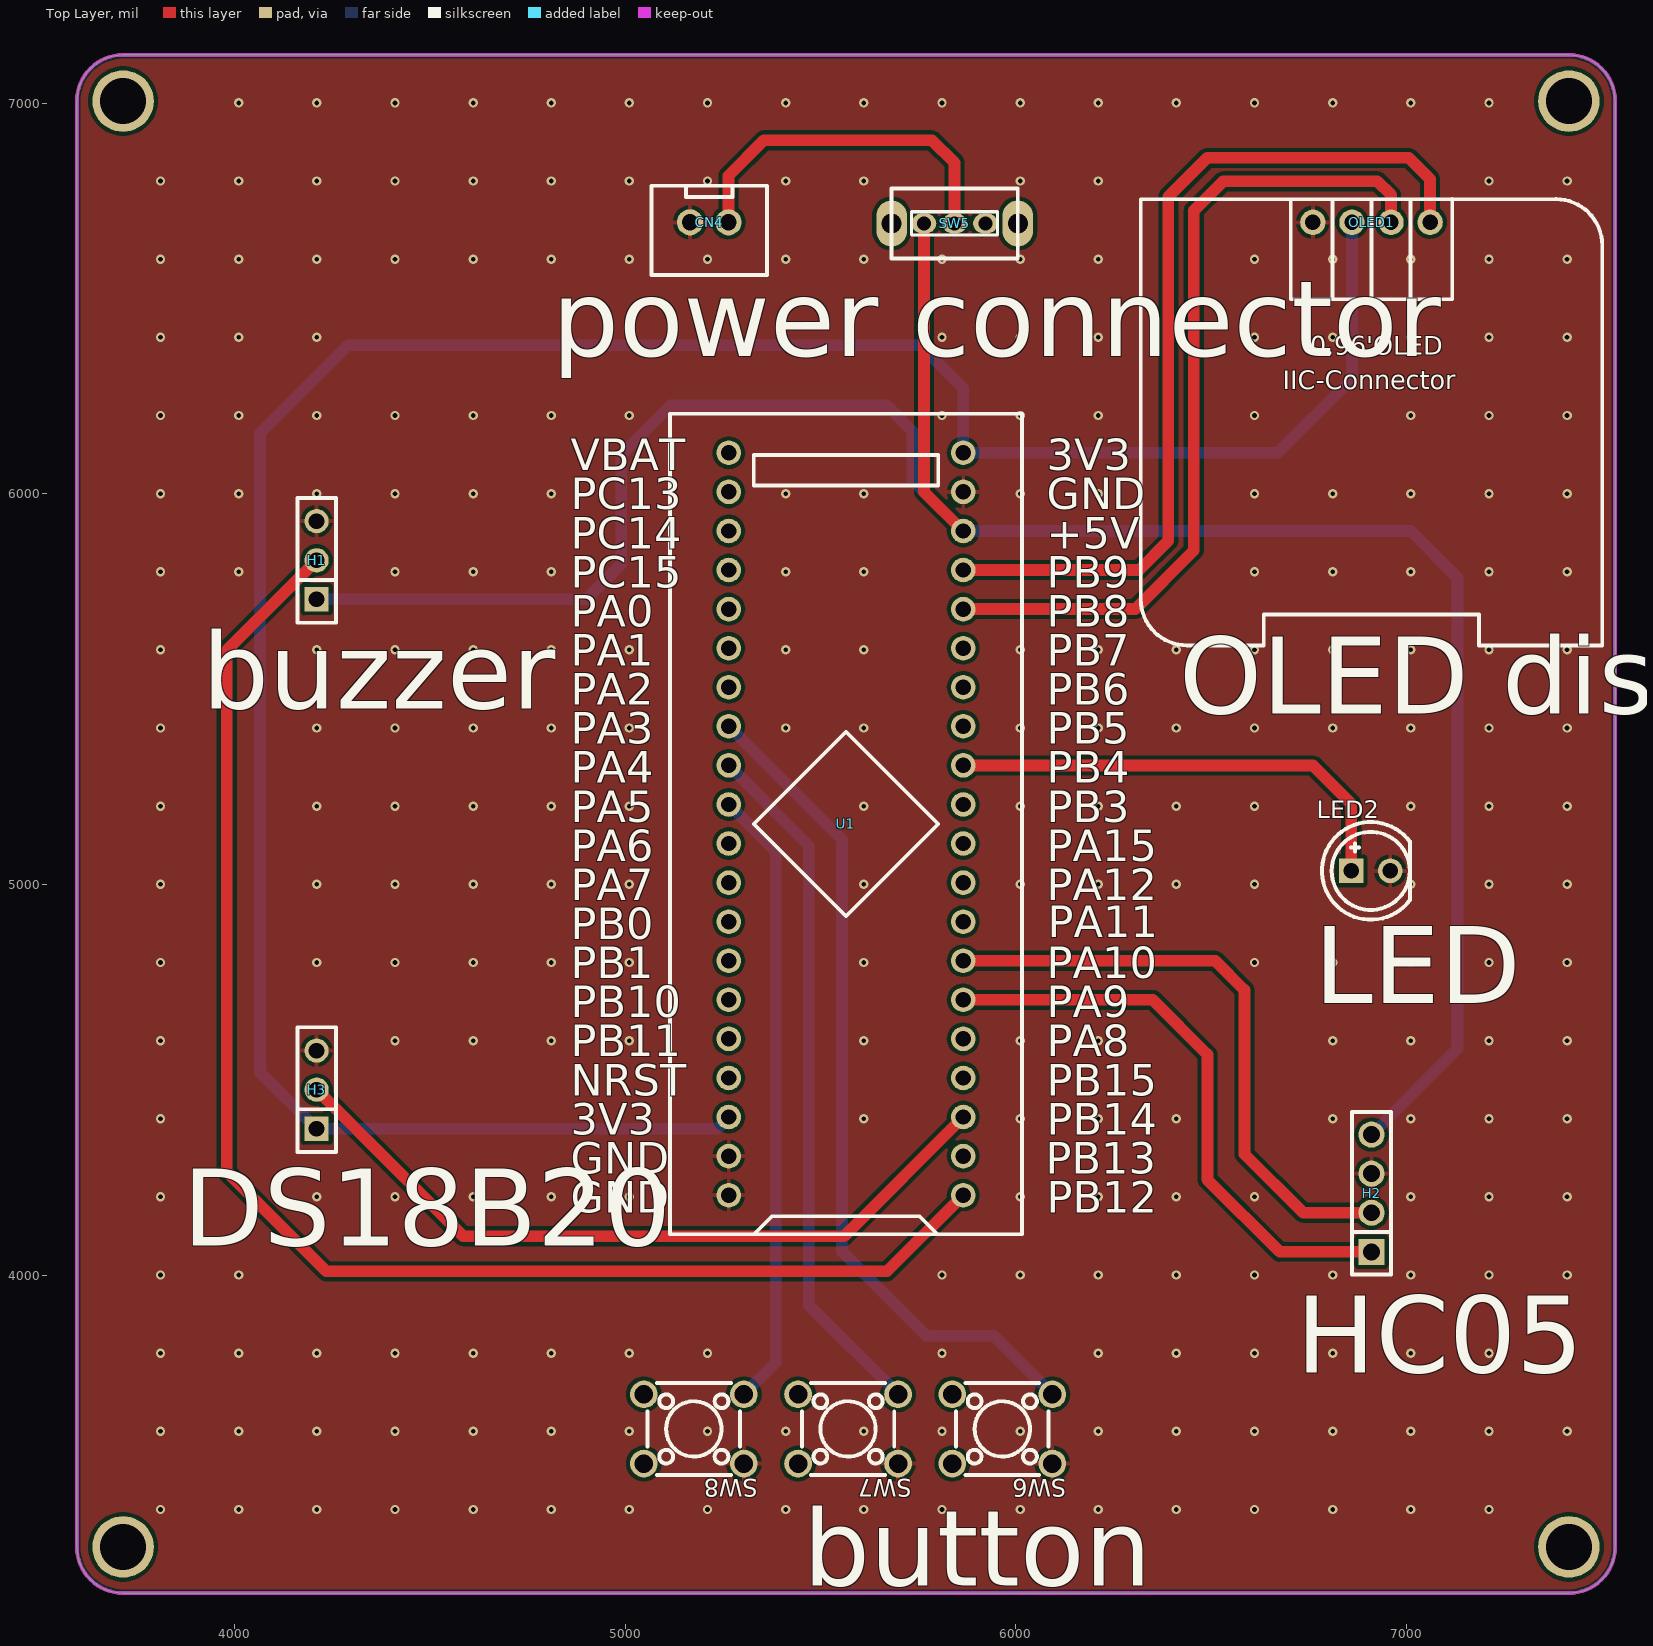
[diagram p0: Top Layer view]
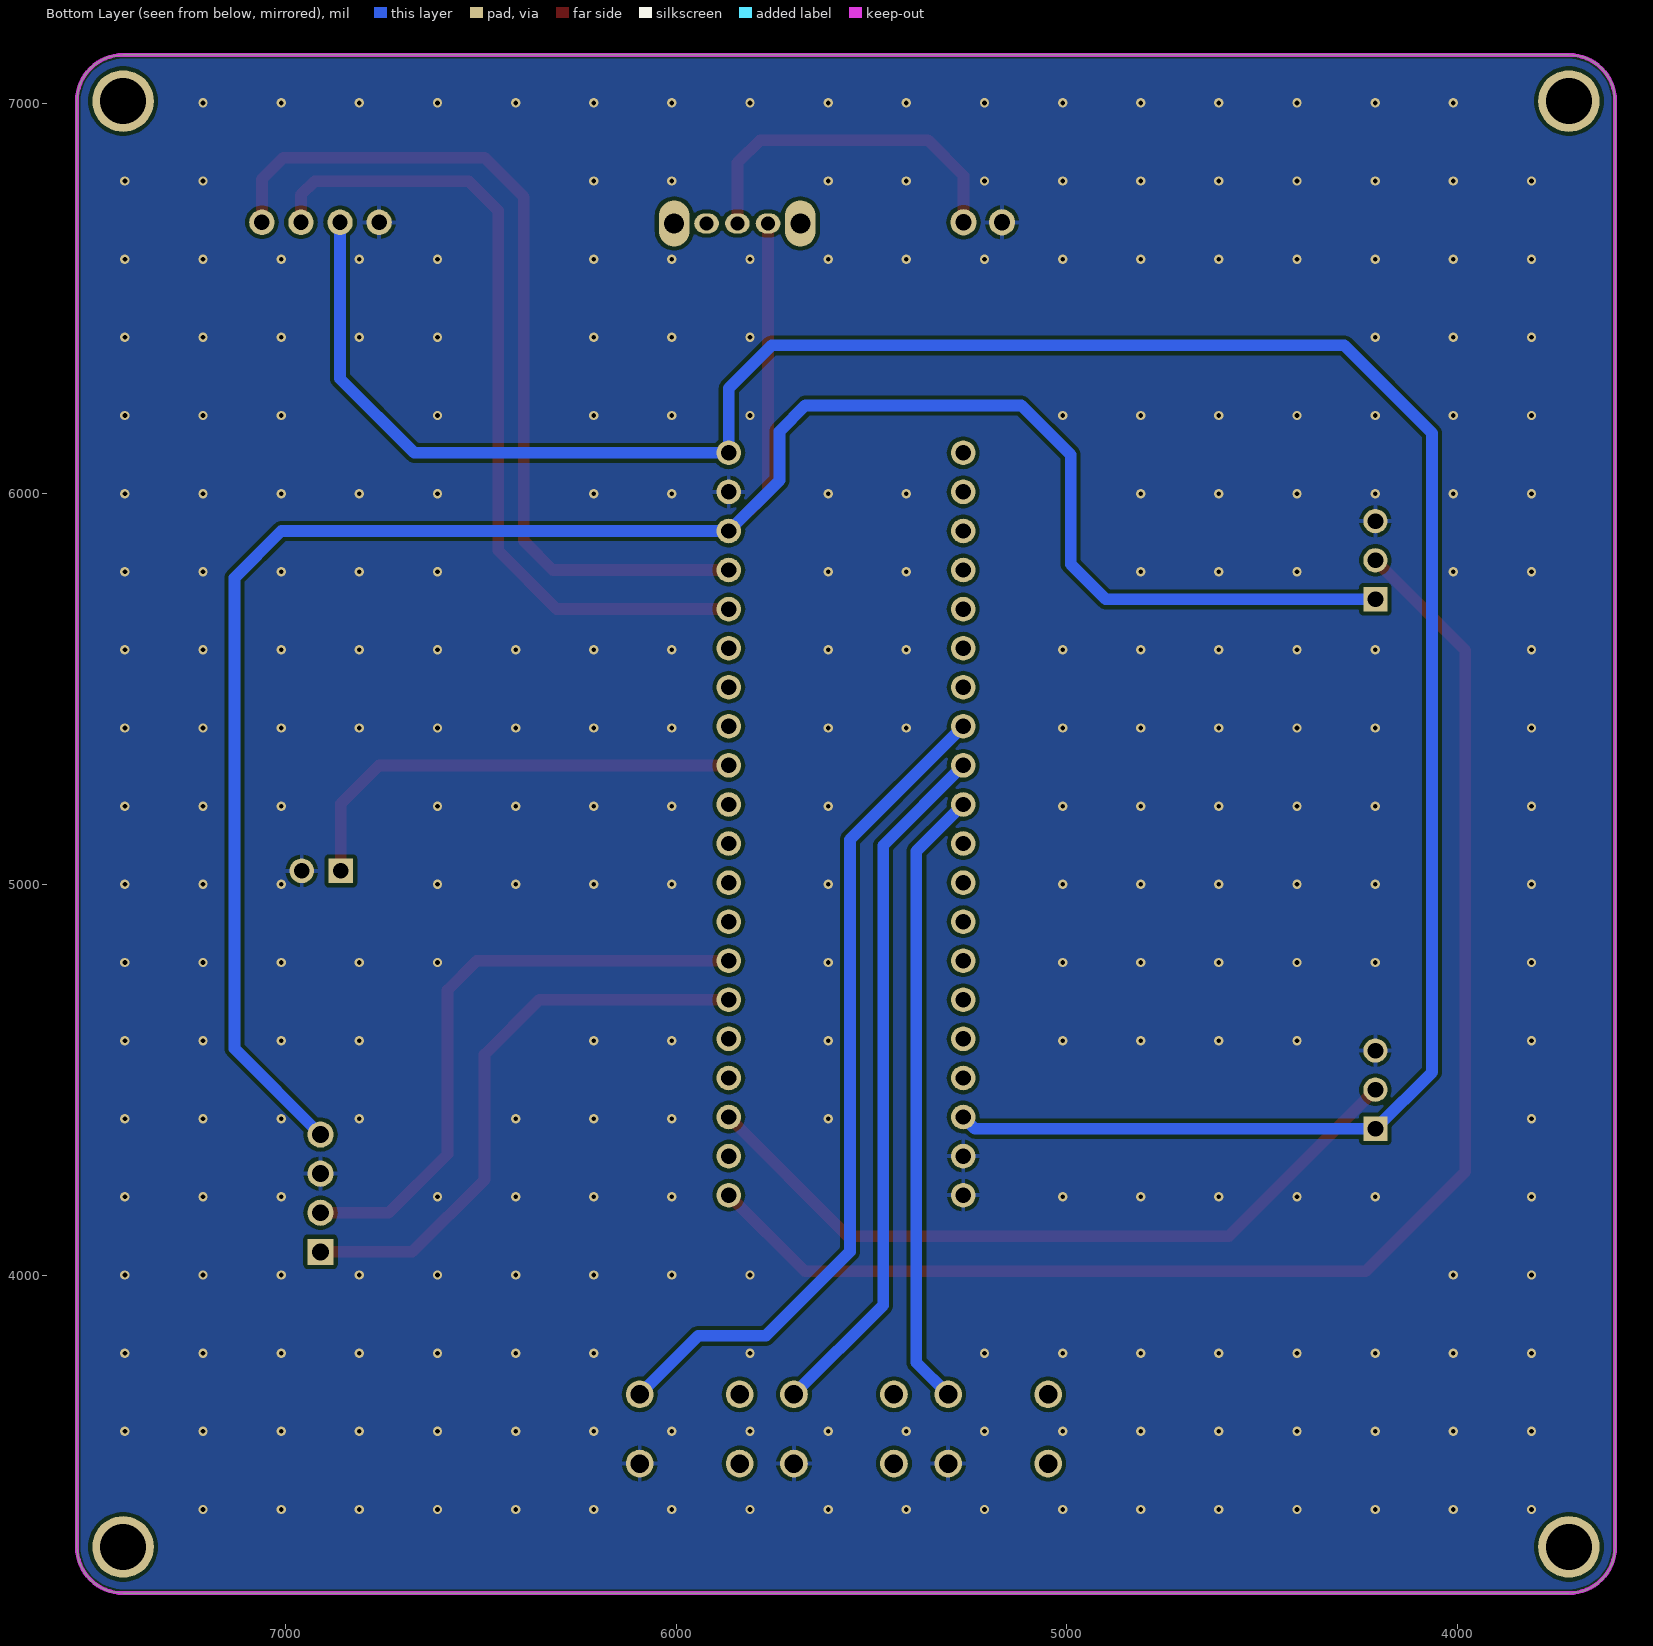
[diagram p1: Bottom Layer view, seen from below]
# Altium PCB MISC89015.pcbdoc
Units mil, origin at the board's own origin, x right, y up, seen from the top; angles counter-clockwise.
Board outline 3937.01 x 3937.01 mil, 2 copper layers (Top Layer, Bottom Layer), stack 62.206 mil thick; 11 components, 38 nets, 79 pads, 271 vias.

## Layer stack, top to bottom
Top Solder Mask Layer: solder mask 0.394, Dk 3.3
Top Layer: signal copper 1.379
Dielectric1: surface 59.449, FR4, Dk 4.5
Bottom Layer: signal copper 1.378
Bottom Solder Mask Layer: solder mask 0.394, Dk 3.3

## Board outline
3714.61,7123.5 ccw(c3714.61,7005.39) 3596.5,7005.39 3596.5,3304.61 ccw(c3714.61,3304.61) 3714.61,3186.5 7415.39,3186.5 ccw(c7415.39,3304.61) 7533.5,3304.61 7533.5,7005.39 ccw(c7415.39,7005.39) 7415.39,7123.5 3714.61,7123.5

## Design rules (kind name [scope] priority, off if disabled: settings)
BoardOutlineClearance copperThickness2oz_1 [All] p2 off: genericclearance=7.99 ignorepadtopadclearanceinfootprint=FALSE except(0: Arc-SplitContinuation Track-SplitContinuation SMDPad-SplitContinuation THPad-SplitContinuation Via-SplitContinuation Fill-SplitContinuation Region-SplitContinuation Poly-SplitContinuation Text-SplitContinuation Hole-SplitContinuation; 5.98: Arc-CutoutEdge Track-CutoutEdge SMDPad-CutoutEdge THPad-CutoutEdge Via-CutoutEdge Text-CutoutEdge; 6.9: Hole-OutlineEdge Hole-CutoutEdge; 10: Poly-OutlineEdge Poly-CutoutEdge; 11.81: Arc-OutlineEdge Track-OutlineEdge SMDPad-OutlineEdge THPad-OutlineEdge Via-OutlineEdge Fill-OutlineEdge Region-OutlineEdge Text-OutlineEdge Fill-CutoutEdge Region-CutoutEdge)
BoardOutlineClearance Plane_innerPlane_1 [All] p4 off: genericclearance=4.02 ignorepadtopadclearanceinfootprint=FALSE except(0: Arc-SplitContinuation Track-SplitContinuation SMDPad-SplitContinuation THPad-SplitContinuation Via-SplitContinuation Fill-SplitContinuation Region-SplitContinuation Poly-SplitContinuation Text-SplitContinuation Hole-SplitContinuation; 5.98: Arc-CutoutEdge Track-CutoutEdge SMDPad-CutoutEdge THPad-CutoutEdge Via-CutoutEdge Text-CutoutEdge; 6.9: Hole-OutlineEdge Hole-CutoutEdge; 10: Poly-OutlineEdge Poly-CutoutEdge; 11.81: Arc-OutlineEdge Track-OutlineEdge SMDPad-OutlineEdge THPad-OutlineEdge Via-OutlineEdge Fill-OutlineEdge Region-OutlineEdge Text-OutlineEdge Fill-CutoutEdge Region-CutoutEdge)
BoardOutlineClearance Copper_copperRegion_1 [All] p6 off: genericclearance=4.02 ignorepadtopadclearanceinfootprint=FALSE except(0: Arc-SplitContinuation Track-SplitContinuation SMDPad-SplitContinuation THPad-SplitContinuation Via-SplitContinuation Fill-SplitContinuation Region-SplitContinuation Poly-SplitContinuation Text-SplitContinuation Hole-SplitContinuation; 5.98: Arc-CutoutEdge Track-CutoutEdge SMDPad-CutoutEdge THPad-CutoutEdge Via-CutoutEdge Text-CutoutEdge; 6.9: Hole-OutlineEdge Hole-CutoutEdge; 10: Poly-OutlineEdge Poly-CutoutEdge; 11.81: Arc-OutlineEdge Track-OutlineEdge SMDPad-OutlineEdge THPad-OutlineEdge Via-OutlineEdge Fill-OutlineEdge Region-OutlineEdge Text-OutlineEdge Fill-CutoutEdge Region-CutoutEdge)
BoardOutlineClearance Copper_copperRegion_copperThickness1oz_1 [All] p8 off: genericclearance=4.02 ignorepadtopadclearanceinfootprint=FALSE except(0: Arc-SplitContinuation Track-SplitContinuation SMDPad-SplitContinuation THPad-SplitContinuation Via-SplitContinuation Fill-SplitContinuation Region-SplitContinuation Poly-SplitContinuation Text-SplitContinuation Hole-SplitContinuation; 5.98: Arc-CutoutEdge Track-CutoutEdge SMDPad-CutoutEdge THPad-CutoutEdge Via-CutoutEdge Text-CutoutEdge; 6.9: Hole-OutlineEdge Hole-CutoutEdge; 10: Poly-OutlineEdge Poly-CutoutEdge; 11.81: Arc-OutlineEdge Track-OutlineEdge SMDPad-OutlineEdge THPad-OutlineEdge Via-OutlineEdge Fill-OutlineEdge Region-OutlineEdge Text-OutlineEdge Fill-CutoutEdge Region-CutoutEdge)
BoardOutlineClearance Copper_copperRegion_Copper_copperRegion_1 [All] p10 off: genericclearance=4.02 ignorepadtopadclearanceinfootprint=FALSE except(0: Arc-SplitContinuation Track-SplitContinuation SMDPad-SplitContinuation THPad-SplitContinuation Via-SplitContinuation Fill-SplitContinuation Region-SplitContinuation Poly-SplitContinuation Text-SplitContinuation Hole-SplitContinuation; 5.98: Arc-CutoutEdge Track-CutoutEdge SMDPad-CutoutEdge THPad-CutoutEdge Via-CutoutEdge Text-CutoutEdge; 6.9: Hole-OutlineEdge Hole-CutoutEdge; 10: Poly-OutlineEdge Poly-CutoutEdge; 11.81: Arc-OutlineEdge Track-OutlineEdge SMDPad-OutlineEdge THPad-OutlineEdge Via-OutlineEdge Fill-OutlineEdge Region-OutlineEdge Text-OutlineEdge Fill-CutoutEdge Region-CutoutEdge)
BoardOutlineClearance copperThickness1oz_1 [All] p12: genericclearance=4.02 ignorepadtopadclearanceinfootprint=FALSE except(0: Arc-SplitContinuation Track-SplitContinuation SMDPad-SplitContinuation THPad-SplitContinuation Via-SplitContinuation Fill-SplitContinuation Region-SplitContinuation Poly-SplitContinuation Text-SplitContinuation Hole-SplitContinuation; 5.98: Arc-CutoutEdge Track-CutoutEdge SMDPad-CutoutEdge THPad-CutoutEdge Via-CutoutEdge Text-CutoutEdge; 6.9: Hole-OutlineEdge Hole-CutoutEdge; 10: Poly-OutlineEdge Poly-CutoutEdge; 11.81: Arc-OutlineEdge Track-OutlineEdge SMDPad-OutlineEdge THPad-OutlineEdge Via-OutlineEdge Fill-OutlineEdge Region-OutlineEdge Text-OutlineEdge Fill-CutoutEdge Region-CutoutEdge)
Clearance copperThickness2oz [All] p1 off: gap=7.99 ignorepadtopadclearanceinfootprint=FALSE except(5.98: SMDPad-Track SMDPad-SMDPad THPad-Track SMDPad-THPad THPad-THPad Track-Via SMDPad-Via THPad-Via Via-Via Fill-SMDPad Region-SMDPad Fill-THPad Region-THPad Fill-Via Region-Via Fill-Fill Fill-Region Region-Region Arc-Track Arc-SMDPad Arc-THPad Arc-Via Fill-Arc Region-Arc Arc-Arc Text-Track SMDPad-Text Text-THPad Text-Via Fill-Text Region-Text Arc-Text Text-Text; 6.9: Hole-Track Hole-SMDPad Hole-THPad Hole-Via Fill-Hole Region-Hole Hole-Arc Hole-Text; 10: Poly-Track Poly-SMDPad Poly-THPad Poly-Via Poly-Fill Poly-Region Poly-Poly Poly-Arc Poly-Text Poly-Hole; 11.81: Fill-Track Region-Track)
Clearance Plane_innerPlane [All] p3 off: gap=4.02 ignorepadtopadclearanceinfootprint=FALSE except(5.98: SMDPad-Track SMDPad-SMDPad THPad-Track SMDPad-THPad THPad-THPad Track-Via SMDPad-Via THPad-Via Via-Via Fill-SMDPad Region-SMDPad Fill-THPad Region-THPad Fill-Via Region-Via Fill-Fill Fill-Region Region-Region Arc-Track Arc-SMDPad Arc-THPad Arc-Via Fill-Arc Region-Arc Arc-Arc Text-Track SMDPad-Text Text-THPad Text-Via Fill-Text Region-Text Arc-Text Text-Text; 6.9: Hole-Track Hole-SMDPad Hole-THPad Hole-Via Fill-Hole Region-Hole Hole-Arc Hole-Text; 10: Poly-Track Poly-SMDPad Poly-THPad Poly-Via Poly-Fill Poly-Region Poly-Poly Poly-Arc Poly-Text Poly-Hole; 11.81: Fill-Track Region-Track)
Clearance Copper_copperRegion [All] p5 off: gap=4.02 ignorepadtopadclearanceinfootprint=FALSE except(5.98: SMDPad-Track SMDPad-SMDPad THPad-Track SMDPad-THPad THPad-THPad Track-Via SMDPad-Via THPad-Via Via-Via Fill-SMDPad Region-SMDPad Fill-THPad Region-THPad Fill-Via Region-Via Fill-Fill Fill-Region Region-Region Arc-Track Arc-SMDPad Arc-THPad Arc-Via Fill-Arc Region-Arc Arc-Arc Text-Track SMDPad-Text Text-THPad Text-Via Fill-Text Region-Text Arc-Text Text-Text; 6.9: Hole-Track Hole-SMDPad Hole-THPad Hole-Via Fill-Hole Region-Hole Hole-Arc Hole-Text; 10: Poly-Track Poly-SMDPad Poly-THPad Poly-Via Poly-Fill Poly-Region Poly-Poly Poly-Arc Poly-Text Poly-Hole; 11.81: Fill-Track Region-Track)
Clearance Copper_copperRegion_copperThickness1oz [All] p7 off: gap=4.02 ignorepadtopadclearanceinfootprint=FALSE except(5.98: SMDPad-Track SMDPad-SMDPad THPad-Track SMDPad-THPad THPad-THPad Track-Via SMDPad-Via THPad-Via Via-Via Fill-SMDPad Region-SMDPad Fill-THPad Region-THPad Fill-Via Region-Via Fill-Fill Fill-Region Region-Region Arc-Track Arc-SMDPad Arc-THPad Arc-Via Fill-Arc Region-Arc Arc-Arc Text-Track SMDPad-Text Text-THPad Text-Via Fill-Text Region-Text Arc-Text Text-Text; 6.9: Hole-Track Hole-SMDPad Hole-THPad Hole-Via Fill-Hole Region-Hole Hole-Arc Hole-Text; 10: Poly-Track Poly-SMDPad Poly-THPad Poly-Via Poly-Fill Poly-Region Poly-Poly Poly-Arc Poly-Text Poly-Hole; 11.81: Fill-Track Region-Track)
Clearance Copper_copperRegion_Copper_copperRegion [All] p9 off: gap=4.02 ignorepadtopadclearanceinfootprint=FALSE except(5.98: SMDPad-Track SMDPad-SMDPad THPad-Track SMDPad-THPad THPad-THPad Track-Via SMDPad-Via THPad-Via Via-Via Fill-SMDPad Region-SMDPad Fill-THPad Region-THPad Fill-Via Region-Via Fill-Fill Fill-Region Region-Region Arc-Track Arc-SMDPad Arc-THPad Arc-Via Fill-Arc Region-Arc Arc-Arc Text-Track SMDPad-Text Text-THPad Text-Via Fill-Text Region-Text Arc-Text Text-Text; 6.9: Hole-Track Hole-SMDPad Hole-THPad Hole-Via Fill-Hole Region-Hole Hole-Arc Hole-Text; 10: Poly-Track Poly-SMDPad Poly-THPad Poly-Via Poly-Fill Poly-Region Poly-Poly Poly-Arc Poly-Text Poly-Hole; 11.81: Fill-Track Region-Track)
Clearance copperThickness1oz [All] p11: gap=4.02 ignorepadtopadclearanceinfootprint=FALSE except(5.98: SMDPad-Track SMDPad-SMDPad THPad-Track SMDPad-THPad THPad-THPad Track-Via SMDPad-Via THPad-Via Via-Via Fill-SMDPad Region-SMDPad Fill-THPad Region-THPad Fill-Via Region-Via Fill-Fill Fill-Region Region-Region Arc-Track Arc-SMDPad Arc-THPad Arc-Via Fill-Arc Region-Arc Arc-Arc Text-Track SMDPad-Text Text-THPad Text-Via Fill-Text Region-Text Arc-Text Text-Text; 6.9: Hole-Track Hole-SMDPad Hole-THPad Hole-Via Fill-Hole Region-Hole Hole-Arc Hole-Text; 10: Poly-Track Poly-SMDPad Poly-THPad Poly-Via Poly-Fill Poly-Region Poly-Poly Poly-Arc Poly-Text Poly-Hole; 11.81: Fill-Track Region-Track)
DiffPairsRouting differentialPair [All] p1: maxlimit=6 minlimit=6 mostfreqgap=6 toplayer_minwidth=5 toplayer_prefwidth=10 toplayer_maxwidth=100 toplayer_mingap=6 toplayer_prefgap=6 toplayer_maxgap=6 bottomlayer_minwidth=5 bottomlayer_prefwidth=10 bottomlayer_maxwidth=100 bottomlayer_mingap=6 bottomlayer_prefgap=6 bottomlayer_maxgap=6 maxuncoupledlength=10
HoleToHoleClearance otherClearance [All] p1: gap=11.81 allowstackedmicrovias=TRUE
Length netLength [All] p1: minlimit=0 maxlimit=0
PasteMaskExpansion pasteMaskExpansion [All] p1: expansion=0
PlaneConnect innerPlane [All] p1: planeconnectstyle=Relief reliefexpansion=20 reliefentries=4 reliefconductorwidth=10 reliefairgap=10
PolygonConnect copperRegion_copperThickness1oz [All] p1 off: connectstyle=Relief reliefconductorwidth=10 reliefentries=4 polygonreliefangle="90 Angle" airgapwidth=10 via.connectstyle=Relief via.reliefconductorwidth=10 via.reliefentries=4 via.polygonreliefangle="90 Angle" via.airgapwidth=10
PolygonConnect copperRegion_Copper_copperRegion [All] p2 off: connectstyle=Relief reliefconductorwidth=10 reliefentries=4 polygonreliefangle="90 Angle" airgapwidth=10 via.connectstyle=Relief via.reliefconductorwidth=10 via.reliefentries=4 via.polygonreliefangle="90 Angle" via.airgapwidth=10
PolygonConnect copperRegion [All] p3: connectstyle=Relief reliefconductorwidth=10 reliefentries=4 polygonreliefangle="90 Angle" airgapwidth=10 via.connectstyle=Relief via.reliefconductorwidth=10 via.reliefentries=4 via.polygonreliefangle="90 Angle" via.airgapwidth=10
RoutingVias viaSize [All] p1: holewidth=12.01 width=24.02 viastyle="Through Hole" minholewidth=11.81 minwidth=19.68 maxholewidth=248.03 maxwidth=393.7
SolderMaskExpansion solderMaskExpansion [IsVia] p1: expansion=-1000 istentingtop=TRUE
SolderMaskExpansion solderMaskExpansion [All] p2: expansion=2 istentingtop=FALSE
Width copperThickness2oz_2 [All] p1 off: maxlimit=100 minlimit=8 preferedwidth=10
Width copperThickness1oz_2 [All] p2: maxlimit=100 minlimit=5 preferedwidth=10

## Components (designator, comment, footprint, x,y, rotation, side; value= is the part's Value field where it differs from the comment)
CN4 "XH2.54*2P_THT" CONN-TH_2P-P2.50-XH2.54-2P 5215,6695 r0 top
H1 "" HDR-TH_3P-P2.54-V-F 4210,5830 r90 top
H2 "" HDR-TH_4P-P2.54-V-F 6910,4210 r90 top
H3 "" HDR-TH_3P-P2.54-V-F 4210,4475 r90 top
LED2 "" LED-TH_5mm 6908.03,5035 r0 top
OLED1 "" 0.96OLED_4P 6910,6695 r0 top
SW5 "" 拨动开关 5837.9,6692.05 r0 top
SW6 "" SW-TH_4P-L6.0-W6.0-P4.50-LS6.5 5965,3606.64 r180 top
SW7 "" SW-TH_4P-L6.0-W6.0-P4.50-LS6.5 5570.29,3606.64 r180 top
SW8 "" SW-TH_4P-L6.0-W6.0-P4.50-LS6.5 5175.57,3606.64 r180 top
U1 "STM32F103C8T6-Card" CONN-TH_L53.3-W22.9_STM32F103C8T6-CARD 5565,5155 r90 top

## Footprints (in the part's own frame and the unit in brackets; to place one, negate y for a bottom-side part, rotate by r counter-clockwise, add the part's x,y. Pads: shape width x height; smd on the part's side, far side on the other; paste and mask are expansions set on the pad)
0.96OLED_4P [mm]
  round 1.65 hole 1 copper offset 0,0: 1(-3.81,-0.001) 2(-1.27,0.002) 3(1.27,0.002) 4(3.81,0.002)
  silkscreen extent -15,-27.5 15,1.5
CONN-TH_2P-P2.50-XH2.54-2P [mm]
  round 1.7 hole 1.05 paste+0 mask+0.05: 1(1.25,0) 2(-1.25,0)
  silkscreen extent -3.75,-3.42 3.75,2.37
CONN-TH_L53.3-W22.9_STM32F103C8T6-CARD [mm]
  round 1.6 hole 1: 1(-24.13,-7.62) 2(-21.59,-7.62) 3(-19.05,-7.62) 4(-16.51,-7.62) 5(-13.97,-7.62) 6(-11.43,-7.62) 7(-8.89,-7.62) 8(-6.35,-7.62) 9(-3.81,-7.62) 10(-1.27,-7.62) 11(1.27,-7.62) 12(3.81,-7.62) 13(6.35,-7.62) 14(8.89,-7.62) 15(11.43,-7.62) 16(13.97,-7.62) 17(16.51,-7.62) 18(19.05,-7.62) 19(21.59,-7.62) 20(24.13,-7.62) 21(24.13,7.62) 22(21.59,7.62) 23(19.05,7.62) 24(16.51,7.62) 25(13.97,7.62) 26(11.43,7.62) 27(8.89,7.62) 28(6.35,7.62) 29(3.81,7.62) 30(1.27,7.62) 31(-1.27,7.62) 32(-3.81,7.62) 33(-6.35,7.62) 34(-8.89,7.62) 35(-11.43,7.62) 36(-13.97,7.62) 37(-16.51,7.62) 38(-19.05,7.62) 39(-21.59,7.62) 40(-24.13,7.62)
  silkscreen extent -26.67,-11.43 26.67,11.43
HDR-TH_3P-P2.54-V-F [mil]
  rect 62x62 hole 40.16: 1(-100,0)
  round 62 hole 40.16: 2(0,0) 3(100,0)
  silkscreen extent -160,-49 160,49
HDR-TH_4P-P2.54-V-F [mm]
  rect 1.7x1.7 hole 1.1: 1(-3.81,0)
  round 1.7 hole 1.1: 2(-1.27,0) 3(1.27,0) 4(3.81,0)
  silkscreen extent -5.29,-1.27 5.29,1.27
LED-TH_5mm [mm]
  rect 1.6x1.6 hole 1 paste+0 mask+0.051: 1(-1.27,0)
  round 1.6 hole 1 paste+0 mask+0.051: 2(1.27,0)
  silkscreen extent -3.17,-3.17 2.54,3.17
SW-TH_4P-L6.0-W6.0-P4.50-LS6.5 [mm]
  round 1.8 hole 1.2: 1(-3.25,2.25) 2(3.25,2.25) 3(-3.25,-2.25) 4(3.25,-2.25)
  silkscreen extent -3,-3 3,3
拨动开关 [mil]
  oval 63x51.2 hole 35.4 paste+0 mask+2: 1(-73.4,0) 2(5,0) 3(84,0)
  oval 78.7x118.1 hole 51.2 paste+0 mask+2: 4(166.7,0) 5(-156.1,0)
  silkscreen extent -156,-90 167,90

## Free pads (board coordinates)
  round 157.48 hole 118.11: 1(3714.61,7005.39) 1(3714.61,3304.61) 1(7415.39,7005.39) 1(7415.39,3304.61)

## Via types
v1: diameter 24.02, hole 12, Top Layer to Bottom Layer, 271 vias

## Nets (pads, with @x,y where several pads share a name; then routed paths per layer and width w, separated by ;. In a path a pad name is that pad's centre, name@x,y a point inside that pad or via, vN(x,y) a via of type N, cw(c..) or ccw(c..) an arc to the next point about the centre after c; other vN are vias at no path point)
$1N17118: CN4.1 SW5.2 | length 914.5
  Top Layer w30: CN4.1 5264.22,6814.22 5355,6905 5785,6905 5842.9,6847.1 SW5.2
+5V: H1.1 H2.4 SW5.1 U1.18 | length 5890.3
  Top Layer w30: SW5.1 5764.5,6005.5 U1.18
  Bottom Layer w30: H1.1 4900,5730 4990,5820 4990,6100 5116.21,6226.21 5668.79,6226.21 5735,6160 5735,6035 U1.18 7010,5905 7130,5785 7130,4580 H2.4
GND: CN4.2 H1.3 H2.3 H3.3 LED2.2 OLED1.1 SW6.1 SW7.1 SW8.1 U1.19 U1.39 U1.40
  other v1: 3810.6,3400.6 4010.6,3400.6 4210.6,3400.6 4410.6,3400.6 4610.6,3400.6 4810.6,3400.6 5010.6,3400.6 5210.6,3400.6 5410.6,3400.6 5610.6,3400.6 5810.6,3400.6 6010.6,3400.6 6210.6,3400.6 6410.6,3400.6 6610.6,3400.6 6810.6,3400.6 7010.6,3400.6 7210.6,3400.6 3810.6,3600.6 4010.6,3600.6 4210.6,3600.6 4410.6,3600.6 4610.6,3600.6 4810.6,3600.6 5010.6,3600.6 5210.6,3600.6 5410.6,3600.6 5610.6,3600.6 5810.6,3600.6 6010.6,3600.6 6210.6,3600.6 6410.6,3600.6 6610.6,3600.6 6810.6,3600.6 7010.6,3600.6 7210.6,3600.6 7410.6,3600.6 3810.6,3800.6 4010.6,3800.6 4210.6,3800.6 4410.6,3800.6 4610.6,3800.6 4810.6,3800.6 5010.6,3800.6 5210.6,3800.6 5810.6,3800.6 6210.6,3800.6 6410.6,3800.6 6610.6,3800.6 6810.6,3800.6 7010.6,3800.6 7210.6,3800.6 7410.6,3800.6 3810.6,4000.6 4010.6,4000.6 5810.6,4000.6 6010.6,4000.6 6210.6,4000.6 6410.6,4000.6 6610.6,4000.6 6810.6,4000.6 7010.6,4000.6 7210.6,4000.6 7410.6,4000.6 3810.6,4200.6 4210.6,4200.6 4410.6,4200.6 4610.6,4200.6 4810.6,4200.6 5010.6,4200.6 6010.6,4200.6 6210.6,4200.6 6410.6,4200.6 6610.6,4200.6 7010.6,4200.6 7210.6,4200.6 7410.6,4200.6 3810.6,4400.6 5610.6,4400.6 6010.6,4400.6 6210.6,4400.6 6410.6,4400.6 6810.6,4400.6 7010.6,4400.6 7210.6,4400.6 7410.6,4400.6 3810.6,4600.6 4410.6,4600.6 4610.6,4600.6 4810.6,4600.6 5010.6,4600.6 5610.6,4600.6 6010.6,4600.6 6210.6,4600.6 6810.6,4600.6 7010.6,4600.6 7210.6,4600.6 7410.6,4600.6 3810.6,4800.6 4210.6,4800.6 4410.6,4800.6 4610.6,4800.6 4810.6,4800.6 5010.6,4800.6 5610.6,4800.6 6610.6,4800.6 6810.6,4800.6 7010.6,4800.6 7210.6,4800.6 7410.6,4800.6 3810.6,5000.6 4210.6,5000.6 4410.6,5000.6 4610.6,5000.6 4810.6,5000.6 5010.6,5000.6 5610.6,5000.6 6010.6,5000.6 6210.6,5000.6 6410.6,5000.6 6610.6,5000.6 7010.6,5000.6 7210.6,5000.6 7410.6,5000.6 3810.6,5200.6 4210.6,5200.6 4410.6,5200.6 4610.6,5200.6 4810.6,5200.6 5010.6,5200.6 5610.6,5200.6 6010.6,5200.6 6210.6,5200.6 6410.6,5200.6 6610.6,5200.6 7010.6,5200.6 7210.6,5200.6 7410.6,5200.6 3810.6,5400.6 4210.6,5400.6 4410.6,5400.6 4610.6,5400.6 4810.6,5400.6 5010.6,5400.6 5410.6,5400.6 5610.6,5400.6 6010.6,5400.6 6210.6,5400.6 6410.6,5400.6 6610.6,5400.6 6810.6,5400.6 7010.6,5400.6 7210.6,5400.6 7410.6,5400.6 3810.6,5600.6 4210.6,5600.6 4410.6,5600.6 4610.6,5600.6 4810.6,5600.6 5010.6,5600.6 5410.6,5600.6 5610.6,5600.6 6010.6,5600.6 6210.6,5600.6 6410.6,5600.6 6610.6,5600.6 6810.6,5600.6 7010.6,5600.6 7210.6,5600.6 7410.6,5600.6 3810.6,5800.6 4010.6,5800.6 4410.6,5800.6 4610.6,5800.6 4810.6,5800.6 5410.6,5800.6 5610.6,5800.6 6610.6,5800.6 6810.6,5800.6 7010.6,5800.6 7210.6,5800.6 7410.6,5800.6 3810.6,6000.6 4010.6,6000.6 4210.6,6000.6 4410.6,6000.6 4610.6,6000.6 4810.6,6000.6 5410.6,6000.6 5610.6,6000.6 6010.6,6000.6 6210.6,6000.6 6610.6,6000.6 6810.6,6000.6 7010.6,6000.6 7210.6,6000.6 7410.6,6000.6 3810.6,6200.6 4010.6,6200.6 4210.6,6200.6 4410.6,6200.6 4610.6,6200.6 4810.6,6200.6 5010.6,6200.6 5810.6,6200.6 6010.6,6200.6 6210.6,6200.6 6610.6,6200.6 7010.6,6200.6 7210.6,6200.6 7410.6,6200.6 3810.6,6400.6 4010.6,6400.6 4210.6,6400.6 5810.6,6400.6 6010.6,6400.6 6210.6,6400.6 6610.6,6400.6 6810.6,6400.6 7010.6,6400.6 7210.6,6400.6 7410.6,6400.6 3810.6,6600.6 4010.6,6600.6 4210.6,6600.6 4410.6,6600.6 4610.6,6600.6 4810.6,6600.6 5010.6,6600.6 5210.6,6600.6 5410.6,6600.6 5610.6,6600.6 5810.6,6600.6 6010.6,6600.6 6210.6,6600.6 6610.6,6600.6 6810.6,6600.6 7010.6,6600.6 7210.6,6600.6 7410.6,6600.6 3810.6,6800.6 4010.6,6800.6 4210.6,6800.6 4410.6,6800.6 4610.6,6800.6 4810.6,6800.6 5010.6,6800.6 5210.6,6800.6 5410.6,6800.6 5610.6,6800.6 6010.6,6800.6 6210.6,6800.6 7210.6,6800.6 7410.6,6800.6 4010.6,7000.6 4210.6,7000.6 4410.6,7000.6 4610.6,7000.6 4810.6,7000.6 5010.6,7000.6 5210.6,7000.6 5410.6,7000.6 5610.6,7000.6 5810.6,7000.6 6010.6,7000.6 6210.6,7000.6 6410.6,7000.6 6610.6,7000.6 6810.6,7000.6 7010.6,7000.6 7210.6,7000.6
NRST: U1.37
PA0: U1.25
PA1: U1.26
PA2: U1.27
PA3: SW6.3 U1.28 | length 2154.2
  Bottom Layer w30: U1.28 5555,5115 5555,4060 5770,3845 5943.17,3845 SW6.3
PA4: SW7.3 U1.29 | length 1789.2
  Bottom Layer w30: U1.29 5470,5100 5470,3923.46 SW7.3
PA5: SW8.3 U1.30 | length 1593.2
  Bottom Layer w30: U1.30 5385,5085 5385,3776.7 SW8.3
PA6: U1.31
PA7: U1.32
PA8: U1.5
PA9: H2.1 U1.6 | length 1499.6
  Top Layer w30: U1.6 6350,4705 6490,4565 6490,4245 6675,4060 H2.1
PA10: H2.2 U1.7 | length 1558.2
  Top Layer w30: U1.7 6510,4805 6585,4730 6585,4310 6735,4160 H2.2
PA11: U1.8
PA12: U1.9
PA15: U1.10
PB0: U1.33
PB1: U1.34
PB3: U1.11
PB4: LED2.1 U1.12 | length 1205.6
  Top Layer w30: U1.12 6760,5305 6858.03,5206.97 LED2.1
PB5: U1.13
PB6: U1.14
PB7: U1.15
PB8: OLED1.3 U1.16 | length 2142.6
  Top Layer w30: U1.16 6305,5705 6455,5855 6455,6725 6530,6800 6925,6800 6960,6765 OLED1.3@6960,6695.05
PB9: OLED1.4 U1.17 | length 2280.2
  Top Layer w30: U1.17 6315,5805 6390,5880 6390,6760 6490,6860 7005,6860 7060,6805 OLED1.4@7060,6695.05
PB10: U1.35
PB11: U1.36
PB12: H1.2 U1.1 | length 3731.7
  Top Layer w30: H1.2 3980,5600 3980,4265 4235,4010 5670,4010 U1.1
PB13: U1.2
PB14: H3.2 U1.3 | length 1936.7
  Top Layer w30: H3.2 4585,4100 5560,4100 U1.3
PB15: U1.4
PC13: U1.22
PC14: U1.23
PC15: U1.24
VBAT: U1.21
VCC: H3.1 OLED1.2 U1.20 U1.38 | length 6485
  Bottom Layer w30: U1.38 5235,4375 H3.1 4065,4520 4065,6155 4290,6380 5755,6380 5865,6270 U1.20 6670,6105 6860,6295 OLED1.2@6860,6695.05
pads on no net: SW5.3 SW5.4 SW5.5 SW6.2 SW6.4 SW7.2 SW7.4 SW8.2 SW8.4

## Polygon pours and split planes (outlines as drawn)
GND on Bottom Layer (solid, remove dead copper, pour order 2): 3525,7245 3525,3080 7700,3080 7700,7245
GND on Top Layer (solid, remove dead copper, pour order 2): 3000,7415 3000,3000 7930,3000 7930,7415

## Keep-outs
Board Outline Layer:
  the board outline again, w10

## Silkscreen, mask and mechanical layers (free items; w line width, h text height)
Top Silkscreen Layer:
  text "power connector" at 4812.87,6351.57 h196.85
  text "VBAT" at 4860.95,6060 h80
  text "3V3" at 6079.16,6060 h80
  text "PC13" at 4860.95,5960 h80
  text "GND" at 6079.16,5960 h80
  text "PC14" at 4860.95,5860 h80
  text "+5V" at 6079.16,5860 h80
  text "PC15" at 4860.95,5760 h80
  text "PB9" at 6079.16,5760 h80
  text "PA0" at 4860.95,5660 h80
  text "PB8" at 6079.16,5660 h80
  text "PA1" at 4860.95,5560 h80
  text "PB7" at 6079.16,5560 h80
  text "PA2" at 4860.95,5460 h80
  text "PB6" at 6079.16,5460 h80
  text "buzzer" at 3916.81,5450 h196.85
  text "OLED display" at 6418.02,5436.57 h196.85
  text "PA3" at 4860.95,5360 h80
  text "PB5" at 6079.16,5360 h80
  text "PA4" at 4860.95,5260 h80
  text "PB4" at 6079.16,5260 h80
  text "PA5" at 4860.95,5160 h80
  text "PB3" at 6079.16,5160 h80
  text "PA6" at 4860.95,5060 h80
  text "PA15" at 6079.16,5060 h80
  text "PA7" at 4860.95,4960 h80
  text "PA12" at 6079.16,4960 h80
  text "PA11" at 6080.95,4865 h80
  text "PB0" at 4860.95,4860 h80
  text "PB1" at 4860.95,4760 h80
  text "PA10" at 6079.16,4760 h80
  text "LED" at 6762.95,4696.57 h196.85
  text "PB10" at 4860.95,4660 h80
  text "PA9" at 6079.16,4660 h80
  text "PB11" at 4860.95,4560 h80
  text "PA8" at 6079.16,4560 h80
  text "NRST" at 4860.95,4460 h80
  text "PB15" at 6079.16,4460 h80
  text "3V3" at 4860.95,4360 h80
  text "PB14" at 6079.16,4360 h80
  text "GND" at 4860.95,4260 h80
  text "PB13" at 6075.95,4260 h80
  text "GND" at 4860.95,4160 h80
  text "PB12" at 6079.16,4160 h80
  text "DS18B20" at 3868.05,4075 h196.85
  text "HC05" at 6717.92,3750 h196.85
  text "button" at 5455,3205 h196.85